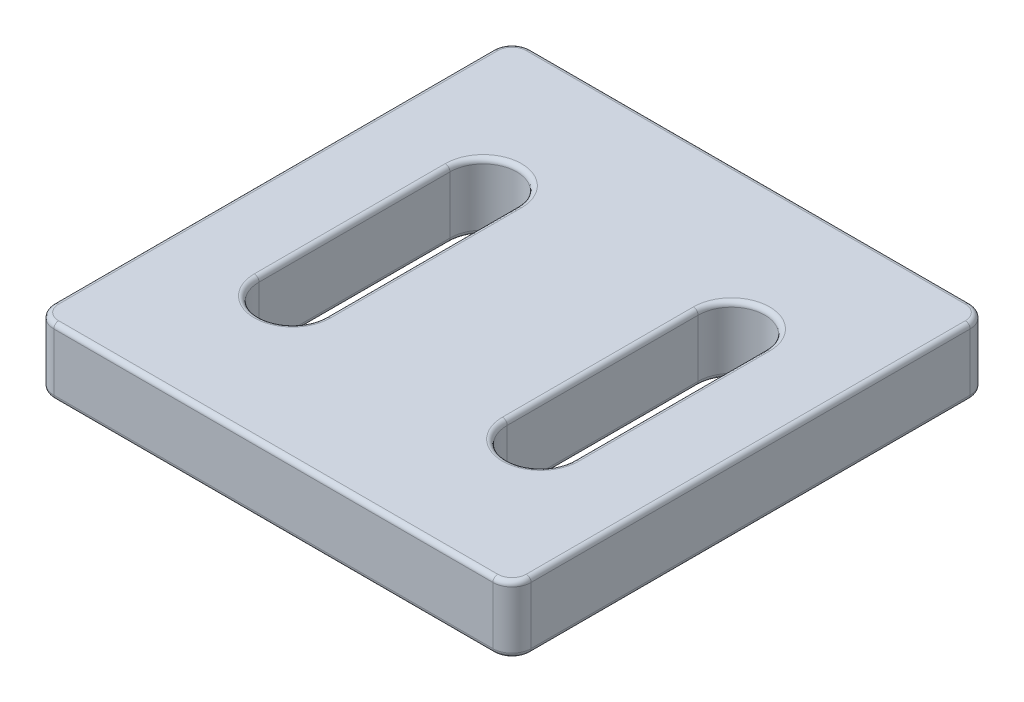
SolidWorks part; units mm, degrees
ref_plane "Front Plane" through (0, 0, 0) normal (0, 0, 1) x (1, 0, 0)
ref_plane "Top Plane" through (0, 0, 0) normal (0, 1, 0) x (1, 0, 0)
ref_plane "Right Plane" through (0, 0, 0) normal (1, 0, 0) x (0, 0, -1)
sketch "Sketch1" plane through (0, 0, 0) normal (0, 1, 0) x (1, 0, 0)
  line L0 (-6.5, -5) -> (-6.5, 5) construction
  line L1 (-11.5, 12.5) -> (11.5, 12.5)
  line L2 (-12.5, 11.5) -> (-12.5, -11.5)
  line L3 (-11.5, -12.5) -> (11.5, -12.5)
  line L4 (12.5, 11.5) -> (12.5, -11.5)
  line L5 (0, -12.5) -> (0, 12.5) construction
  line L6 (-12.5, 0) -> (12.5, 0) construction
  line L7 (-8.25, -5) -> (-8.25, 5)
  line L8 (-4.75, -5) -> (-4.75, 5)
  line L9 (6.5, -5) -> (6.5, 5) construction
  line L10 (8.25, -5) -> (8.25, 5)
  line L11 (4.75, -5) -> (4.75, 5)
  arc A0 (-11.5, 12.5) -> (-12.5, 11.5) centre (-11.5, 11.5) ccw
  arc A1 (11.5, 12.5) -> (12.5, 11.5) centre (11.5, 11.5) cw
  arc A2 (11.5, -12.5) -> (12.5, -11.5) centre (11.5, -11.5) ccw
  arc A3 (-12.5, -11.5) -> (-11.5, -12.5) centre (-11.5, -11.5) ccw
  arc A4 (-8.25, -5) -> (-4.75, -5) centre (-6.5, -5) ccw
  arc A5 (-4.75, 5) -> (-8.25, 5) centre (-6.5, 5) ccw
  arc A6 (8.25, -5) -> (4.75, -5) centre (6.5, -5) cw
  arc A7 (4.75, 5) -> (8.25, 5) centre (6.5, 5) cw
  point P0 (0, 0)
  point P6 (-12.5, 12.5)
  point P9 (12.5, 12.5)
  point P15 (-12.5, -12.5)
  point P18 (-6.5, 0)
  point P25 (6.5, 0)
  dimension "D3" = 1
  dimension "D1" = 25
  dimension "D2" = 25
  dimension "D4" = 6.5
  dimension "D5" = 3.5
  dimension "D6" = 10
extrude "Boss-Extrude1" add sketch "Sketch1" along normal blind 3.5
fillet "Fillet1" radius 0.25 32 edges at (4.75, 0, 0) (6.5, 0, -6.75) (8.25, 0, 0) (6.5, 0, 6.75) (-12.5, 0, 0) (-12.2071, 0, 12.2071) (0, 0, 12.5) (12.2071, 0, 12.2071) (12.5, 0, 0) (12.2071, 0, -12.2071) (0, 0, -12.5) (-12.2071, 0, -12.2071) (-8.25, 0, 0) (-6.5, 0, -6.75) (-4.75, 0, 0) (-6.5, 0, 6.75) (6.5, 3.5, -6.75) (4.75, 3.5, 0) (6.5, 3.5, 6.75) (8.25, 3.5, 0) (-6.5, 3.5, -6.75) (-8.25, 3.5, 0) (-6.5, 3.5, 6.75) (-4.75, 3.5, 0) (0, 3.5, -12.5) (12.2071, 3.5, -12.2071) (12.5, 3.5, 0) (12.2071, 3.5, 12.2071) (0, 3.5, 12.5) (-12.2071, 3.5, 12.2071) (-12.5, 3.5, 0) (-12.2071, 3.5, -12.2071)
